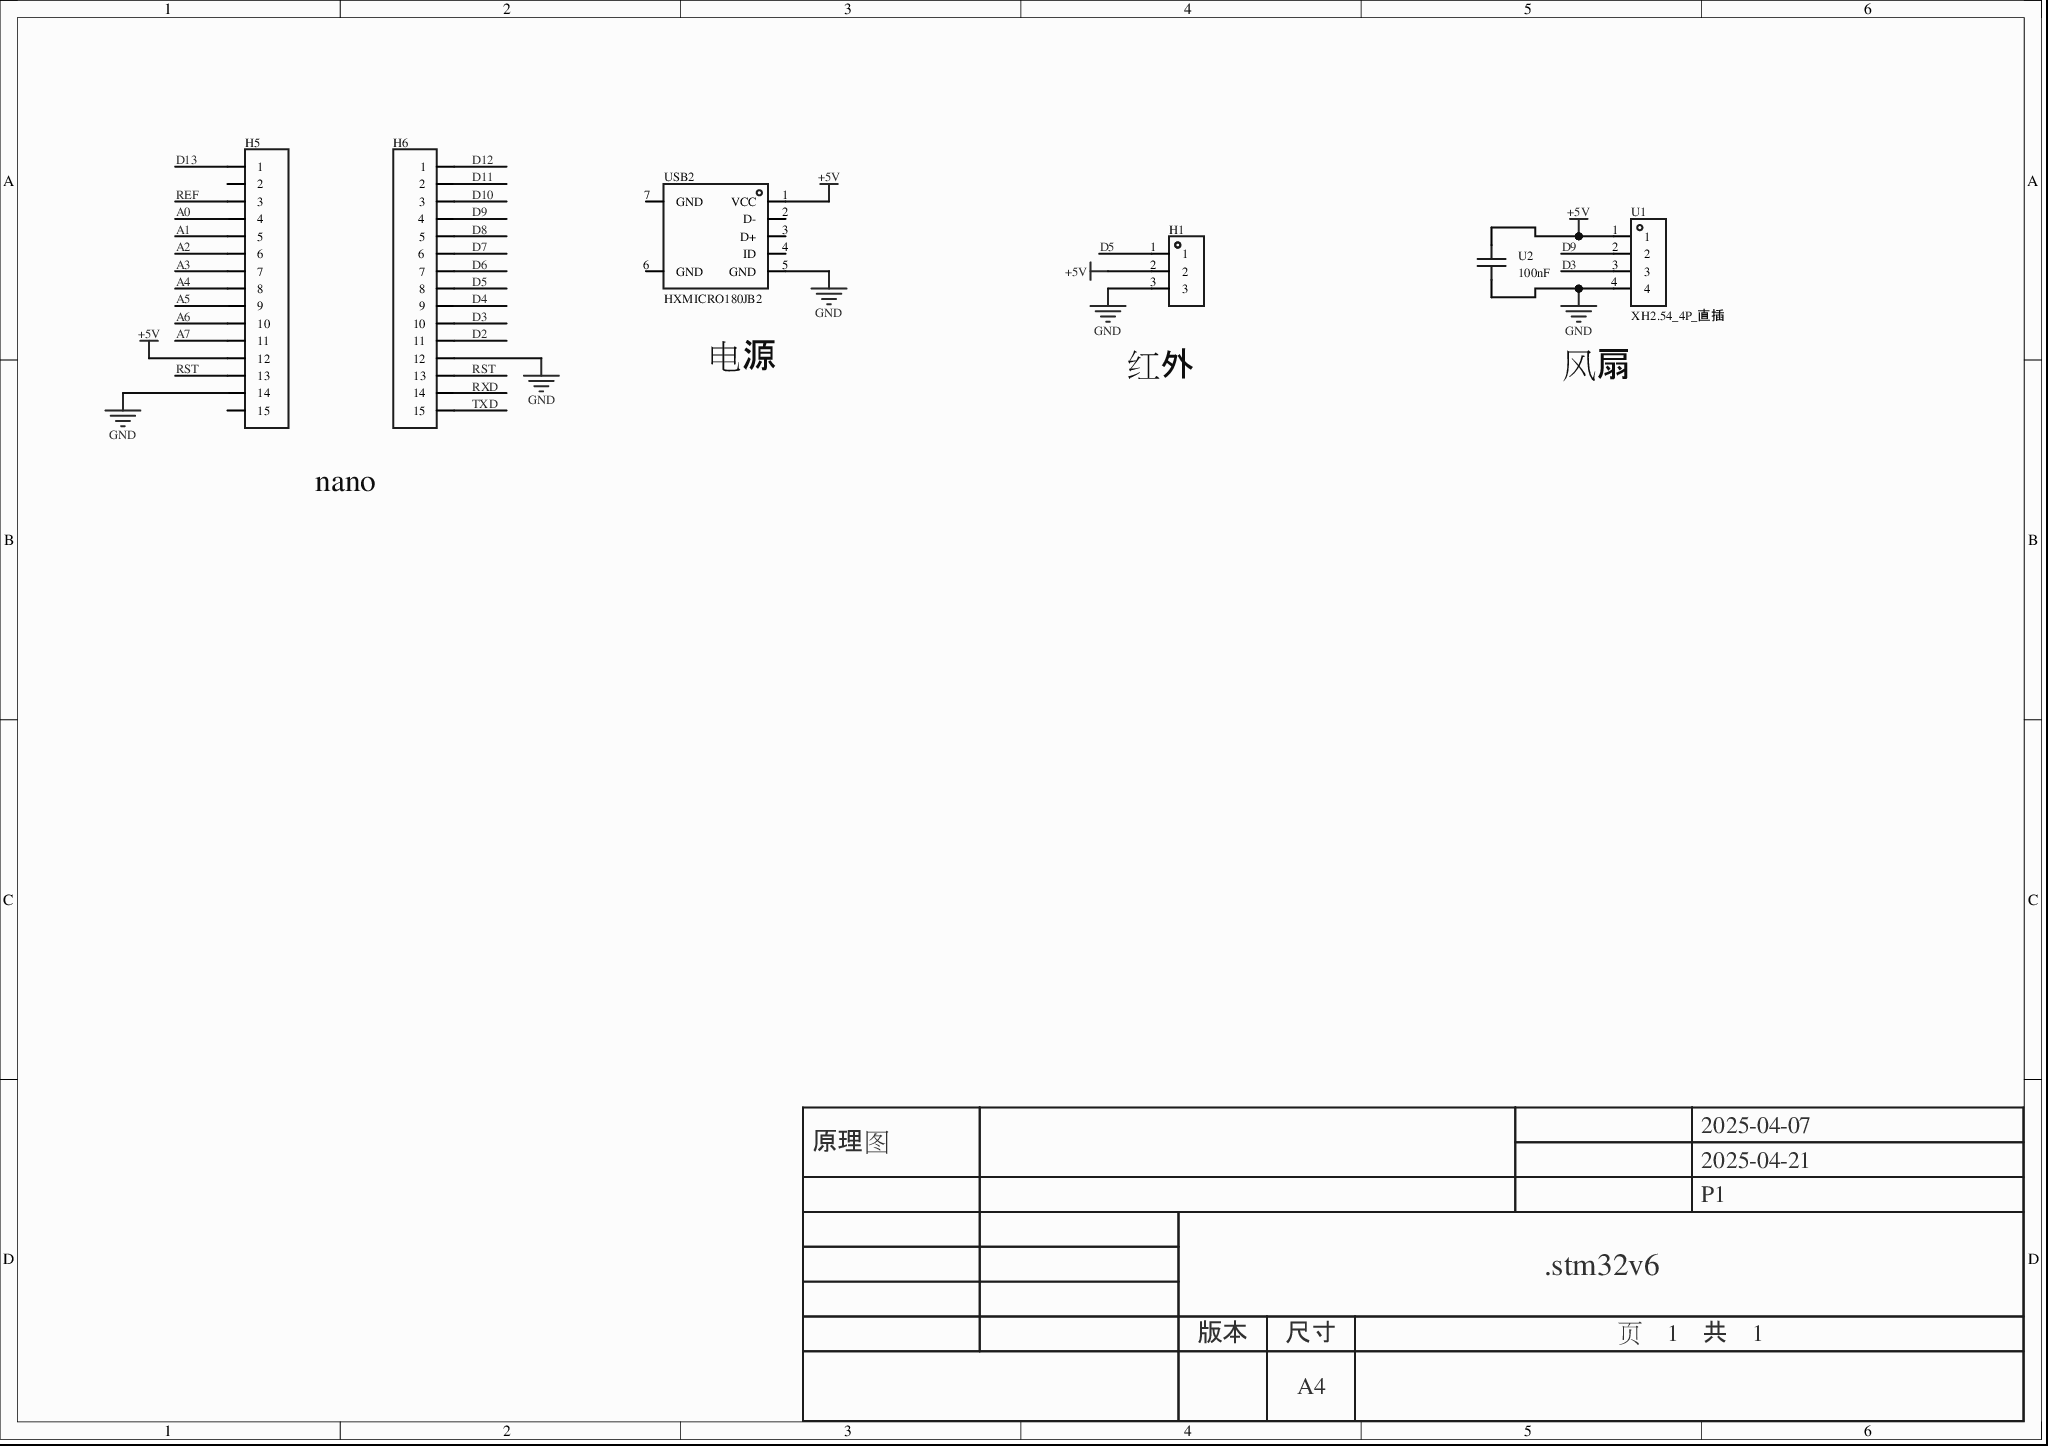
[diagram p0: MISC52018-3.schdoc]
# Altium project MISC52018-2.PrjPcb
1 sheet, 6 parts. Net scope: global (net labels, ports and power ports of the same name join across sheets).
Board file: MISC52018.pcbdoc

## Sheet MISC52018-3.schdoc
size 297 x 209 mm; Version: V1.0; @Project Name: MISC52018; @Page Count: 1; @Update Date: 2026-05-02; @Create Date: 2026-05-02; @Schematic Name: MISC52018; @Page No: 1; @Create Time: 23:22:16; @Update Time: 17:32:40; @Board Name: MISC52018

### Parts
H1  (no value)  [HDR-TH_3P-P2.54-V-F]
H5  (no value)  [HDR-TH_15P-P2.54-V-F-1]
H6  (no value)  [HDR-TH_15P-P2.54-V-F-1]
U1  XH2.54_4P_直插  [CONN-TH_4P-P2.50-XH2.54-4P]
U2  100nF  [CAP-TH_L5.0-W2.5-P5.00-D1.0]
USB2  HXMICRO180JB2  [MICRO-USB-TH_HXMICRO180JB2]

### Nets
+5V: H1.2 H5.12 U1.1 U2.1 USB2.1(VCC)
GND: H1.3 H5.14 H6.12 U1.4 U2.2 USB2.5(GND)
A0: H5.4
A1: H5.5
A2: H5.6
A3: H5.7
A4: H5.8
A5: H5.9
A6: H5.10
A7: H5.11
D2: H6.11
D3: H6.10 U1.3
D4: H6.9
D5: H1.1 H6.8
D6: H6.7
D7: H6.6
D8: H6.5
D9: H6.4 U1.2
D10: H6.3
D11: H6.2
D12: H6.1
D13: H5.1
REF: H5.3
RST: H5.13 H6.13
RXD: H6.14
TXD: H6.15

Not connected (* = marked no-connect by the designer): H5 2 15; USB2 2(D-) 3(D+) 4(ID) 6(GND) 7(GND)

### Notes on the sheet
- 电源
- (near H1) 红外
- 风扇
- nano
- 2025-04-07
- 原理图
- 2025-04-21
- P1
- .stm32v6
- 版本
- 尺寸
- A4
- 页    1    共    1

### Library data of the parts
H1 = HDR-F_2.54_1x3P: Symbol: PM254V-11-03-H85; 3D Model: f3b3cc5aae9641bf9e56fc160cef875b; 3D Model Transform: 299.9994,100,0,0,0,0,0,0,-118.11; ConvertToPcb: yes; ModelName: HDR2.54-F-LI-1X3P; Device: HDR-F_2.54_1x3P; Supplier Part: C541850; Supplier Footprint: 插件; AddInBom: yes; FootprintName: HDR-TH_3P-P2.54-V-F
H5 H6 = HDR-F_2.54_1x15P: ConvertToPcb: yes; ModelId: 88d88d3d05774da49ce8fa2ce222e7100819f05c4eef4c71ace90d822a990e87; ModelTransform: 1515.745,94.488,0,0,0,0,0,0,-125.984; Symbol: HDR-F_2.54_1x15P; Device: HDR-F_2.54_1x15P; AddInBom: yes; SupplierPart: C124408; Supplier Footprint: 插件,; FootprintName: HDR-TH_15P-P2.54-V-F-1; ModelName: HDR-TH_15P-P2.54-V-F-1
U1 = XH2.54_4P_直插: 3D Model: c69236e4c0a047c6aeeeefc1552045f50819f05c4eef4c71ace90d822a990e87; 3D Model Transform: 492.125,228.346,0,180,0,0,0,-19.685,-137.795; AddInBom: yes; Symbol: XH2.54_4P_直插; Device: XH2.54_4P_直插; LCSC Part Name: XH2.54_4P_直插; Supplier Part: C9900008616; Manufacturer Part: XH2.54_4P_直插; Supplier Footprint: XH2.54_4P; JLCPCB Part Class: Extended Part; Supplier: LCSC; ConvertToPcb: yes; FootprintName: CONN-TH_4P-P2.50-XH2.54-4P; ModelName: CONN-TH_4P-P2.50-XH2.54-4P
U2 = 100nF: Symbol: 100NF_C9900015256; 3D Model: 08e3d7481fc7486bb1b263873f51e1e10819f05c4eef4c71ace90d822a990e87; 3D Model Transform: 224.652,98.425,0,0,0,0,-0.005,0,-137.795; AddInBom: yes; ModelName: CAP-TH_BD5.0-W2.5-P5.08; Device: 100nF; LCSC Part Name: 100nF; Supplier Part: C9900015256; Manufacturer Part: 100nF; Supplier Footprint: CAP-TH_L5.0-W2.5-P5.00-D1.0; JLCPCB Part Class: Extended Part; Supplier: LCSC; ConvertToPcb: yes; FootprintName: CAP-TH_L5.0-W2.5-P5.00-D1.0
USB2 = HXMICRO180JB2: 3D Model: 32b85b123c6e4ce58522a70e58ed963c0819f05c4eef4c71ace90d822a990e87; 3D Model Transform: 316.06626,114.173,0,0,0,0,0,8.504,-59.055; AddInBom: yes; Symbol: HXMICRO180JB2; Device: HXMICRO180JB2; LCSC Part Name: HXMICRO180JB2; Supplier Part: C9900088445; Manufacturer Part: HXMICRO180JB2; Supplier Footprint: MicroUSB母座; JLCPCB Part Class: Extended Part; Supplier: LCSC; ConvertToPcb: yes; FootprintName: MICRO-USB-TH_HXMICRO180JB2; ModelName: MICRO-USB-TH_HXMICRO180JB2